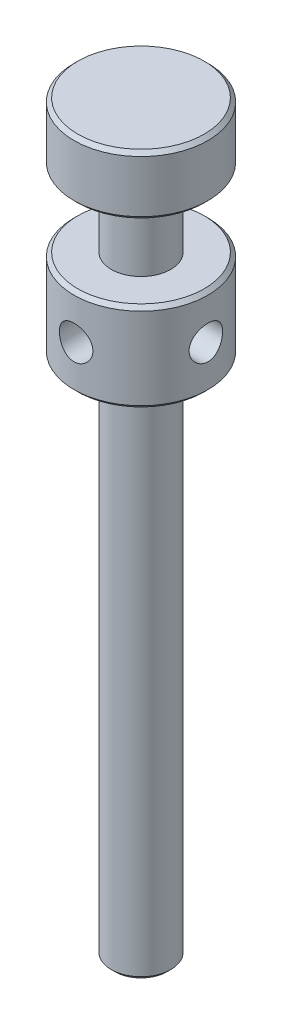
SolidWorks part; units mm, degrees
ref_plane "Front Plane" through (0, 0, 0) normal (0, 0, 1) x (1, 0, 0)
ref_plane "Top Plane" through (0, 0, 0) normal (0, 1, 0) x (1, 0, 0)
ref_plane "Right Plane" through (0, 0, 0) normal (1, 0, 0) x (0, 0, -1)
sketch "Sketch1" plane through (0, 0, 0) normal (0, 1, 0) x (1, 0, 0)
  circle A0 centre (0, 0) radius 4
  dimension "D1" = 8
extrude "Boss-Extrude1" add sketch "Sketch1" along normal blind 10
sketch "Sketch2" plane through (0, 10, 0) normal (0, 1, 0) x (1, 0, 0)
  circle A0 centre (0, 0) radius 9
  dimension "D1" = 18
extrude "Boss-Extrude2" add sketch "Sketch2" along normal blind 8
sketch "Sketch3" plane through (0, 0, 0) normal (0, -1, 0) x (1, 0, 0)
  circle A0 centre (0, 0) radius 9
  circle A1 centre (0, 0) radius 9 construction
extrude "Boss-Extrude3" add sketch "Sketch3" along normal blind 12
sketch "Sketch4" plane through (0, -12, 0) normal (0, -1, 0) x (1, 0, 0)
  circle A0 centre (0, 0) radius 4
  dimension "D1" = 8
extrude "Boss-Extrude4" add sketch "Sketch4" along normal blind 70
cosmetic thread "Cosmetic Thread1" parameters "D1"=60, "D2"=6.8
chamfer "Chamfer1" distance 0.5 angle 45 1 edges at (0, -82, -4)
sketch "Sketch6" plane through (0, 0, 0) normal (0, 0, 1) x (1, 0, 0)
  line L0 (9, 0) -> (-9, 0) construction
  circle A0 centre (0, -6) radius 2.25
  dimension "D1" = 4.5
  dimension "D2" = 6
extrude "Cut-Extrude2" cut sketch "Sketch6" against normal blind 10
pattern_circular "CirPattern1" count 4 over 360 about axis through (0, 18, 0) along (0, -1, 0) of "Cut-Extrude2"
chamfer "Chamfer2" distance 0.5 angle 45 4 edges at (0, 18, 9) (0, -12, -9) (0, 0, -9) (0, 10, 9)
